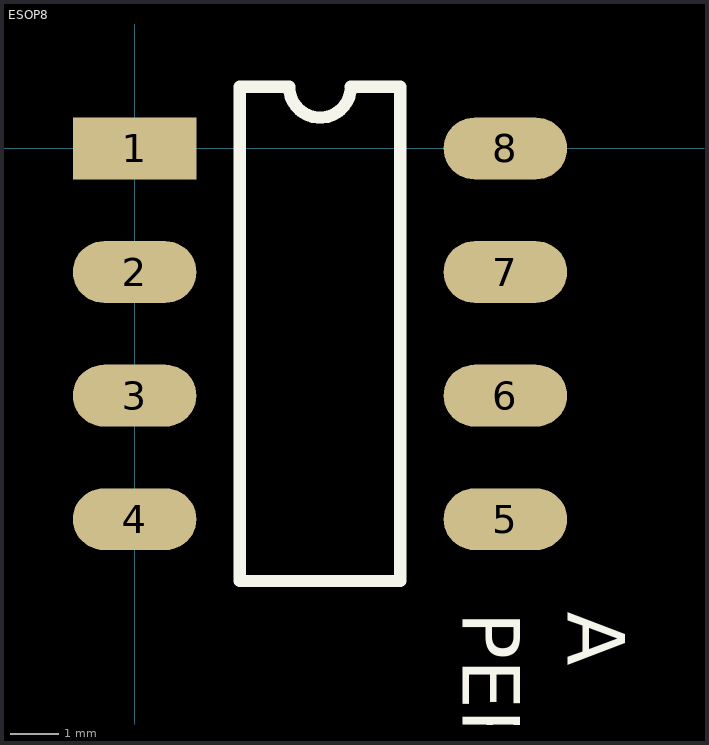
[diagram p0: the footprint, top view; thin cyan lines are the x and y axes]
# Altium footprint library MISC84315-4.PcbLib: 1 footprints
Each footprint in its own frame and in the unit in brackets; x right, y up, seen from the top. Pads: shape width x height; smd on the part's side, far side on the other; paste and mask are expansions set on the pad; w line width, h text height; cw(c..) or ccw(c..) is an arc to the next point about the centre after c.

## ESOP8 [mil]
pads (8):
  rect 100x50 smd: 1(0,0)
  oval 100x50 smd: 2(0,-100) 3(0,-200) 4(0,-300) 5(300,-300) 6(300,-200) 7(300,-100) 8(300,0)
Top Overlay:
  lines w10: 85,-350 85,50 125,50 ccw(c150,50) 175,50 215,50 215,-350 85,-350
  text "A" at 335,-375 h80
  text "PERSON" at 250,-375 h80